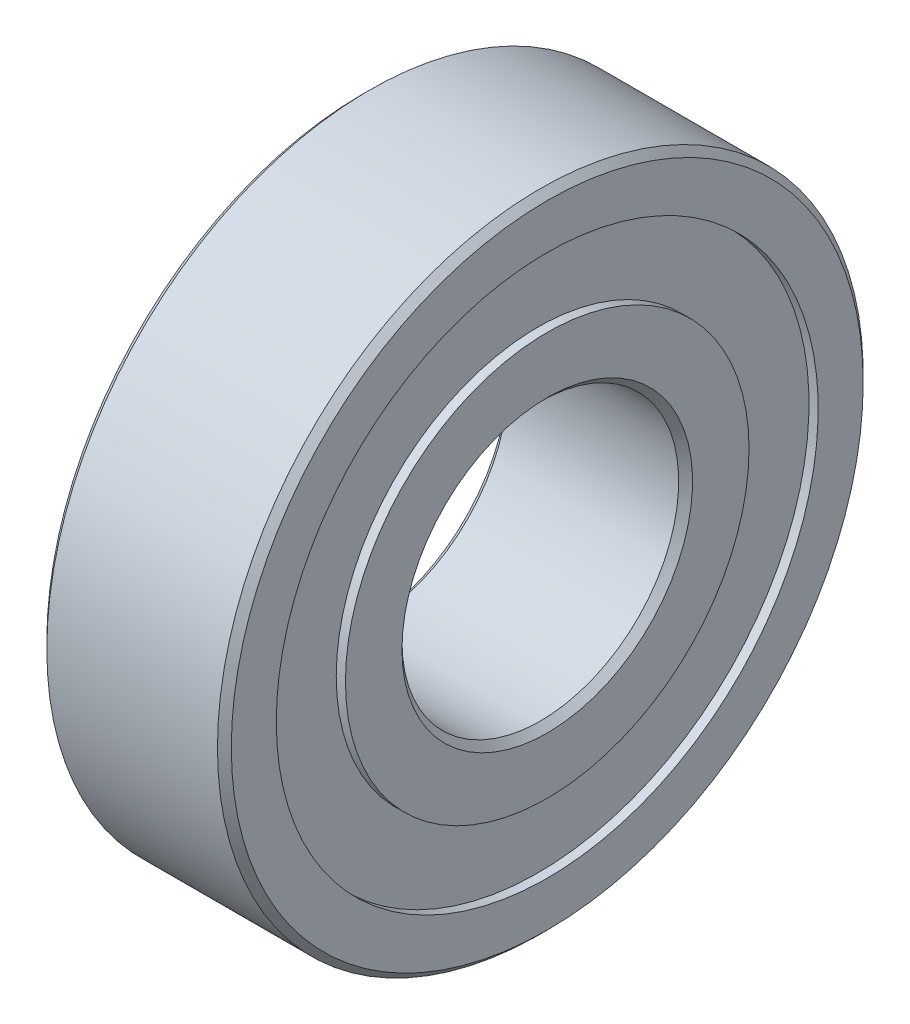
from build123d import *


with BuildPart() as part:
    # 草图1 → 旋转1 (revolve)
    with BuildSketch(Plane.XY, mode=Mode.PRIVATE) as revolve_1_sk:
        Polygon((-4, 13.7), (-4, 11.75), (-3.6, 11.75), (-3.6, 8.75), (-4, 8.75), (-4, 6.3), (-3.7, 6), (3.7, 6), (4, 6.3), (4, 8.75), (3.6, 8.75), (3.6, 11.75), (4, 11.75), (4, 13.7), (3.7, 14), (-3.7, 14), align=None)
    revolve(revolve_1_sk.sketch.rotate(Axis((4, 0, 0), (-1, 0, 0)), 270), axis=Axis((4, 0, 0), (-1, 0, 0)))


solid = part.part
